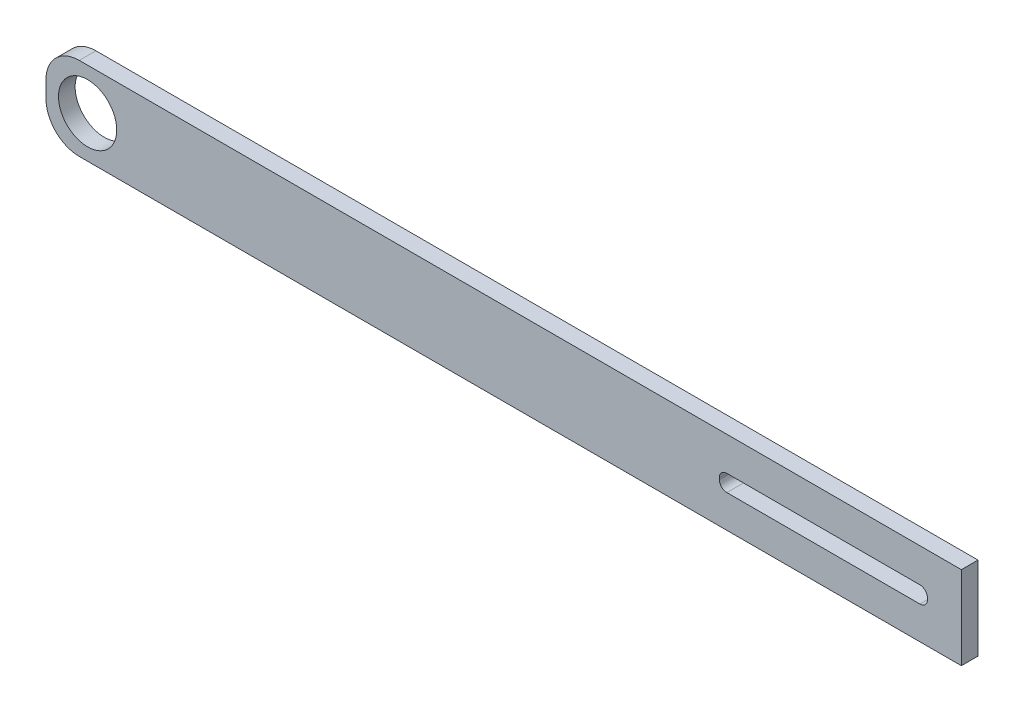
from build123d import *

# Parameters (mm, degrees)
SKETCH1_W           = 550
SKETCH1_H           = 50
BOSS_EXTRUDE1_DEPTH = 10
SKETCH2_R           = 17.5
CUT_EXTRUDE1_DEPTH  = 10
CUT_EXTRUDE2_DEPTH  = 10
FILLET1_R           = 20


with BuildPart() as part:
    # Sketch1 → Boss-Extrude1 (new body)
    with BuildSketch(Plane.XY):
        Rectangle(SKETCH1_W, SKETCH1_H)
    extrude(amount=BOSS_EXTRUDE1_DEPTH)

    # Sketch2 → Cut-Extrude1 (cut)
    with BuildSketch(Plane.XY.offset(10)):
        with Locations((-250, 0)):
            Circle(SKETCH2_R)
    extrude(amount=-CUT_EXTRUDE1_DEPTH, mode=Mode.SUBTRACT)

    # Sketch3 → Cut-Extrude2 (cut)
    with BuildSketch(Plane.XY.offset(10)):
        with BuildLine():
            Line((250.099813904, -5.340973555), (134.099813904, -5.340973555))
            ThreePointArc((134.099813904, -5.340973555), (130.917833389, -4.02295407), (129.599813904, -0.840973555))
            Line((129.599813904, -0.840973555), (129.599813904, 0.159026445))
            ThreePointArc((129.599813904, 0.159026445), (130.917833389, 3.341006961), (134.099813904, 4.659026445))
            Line((134.099813904, 4.659026445), (250.099813904, 4.659026445))
            ThreePointArc((250.099813904, 4.659026445), (253.281794419, 3.341006961), (254.599813904, 0.159026445))
            Line((254.599813904, 0.159026445), (254.599813904, -0.840973555))
            ThreePointArc((254.599813904, -0.840973555), (253.281794419, -4.02295407), (250.099813904, -5.340973555))
        make_face()
    extrude(amount=-CUT_EXTRUDE2_DEPTH, mode=Mode.SUBTRACT)

    # Fillet1
    fillet1_edges = [part.edges().sort_by_distance(p)[0] for p in [
        (-275, 25, 5),
        (-275, -25, 5),
    ]]
    fillet(fillet1_edges, radius=FILLET1_R)


solid = part.part
